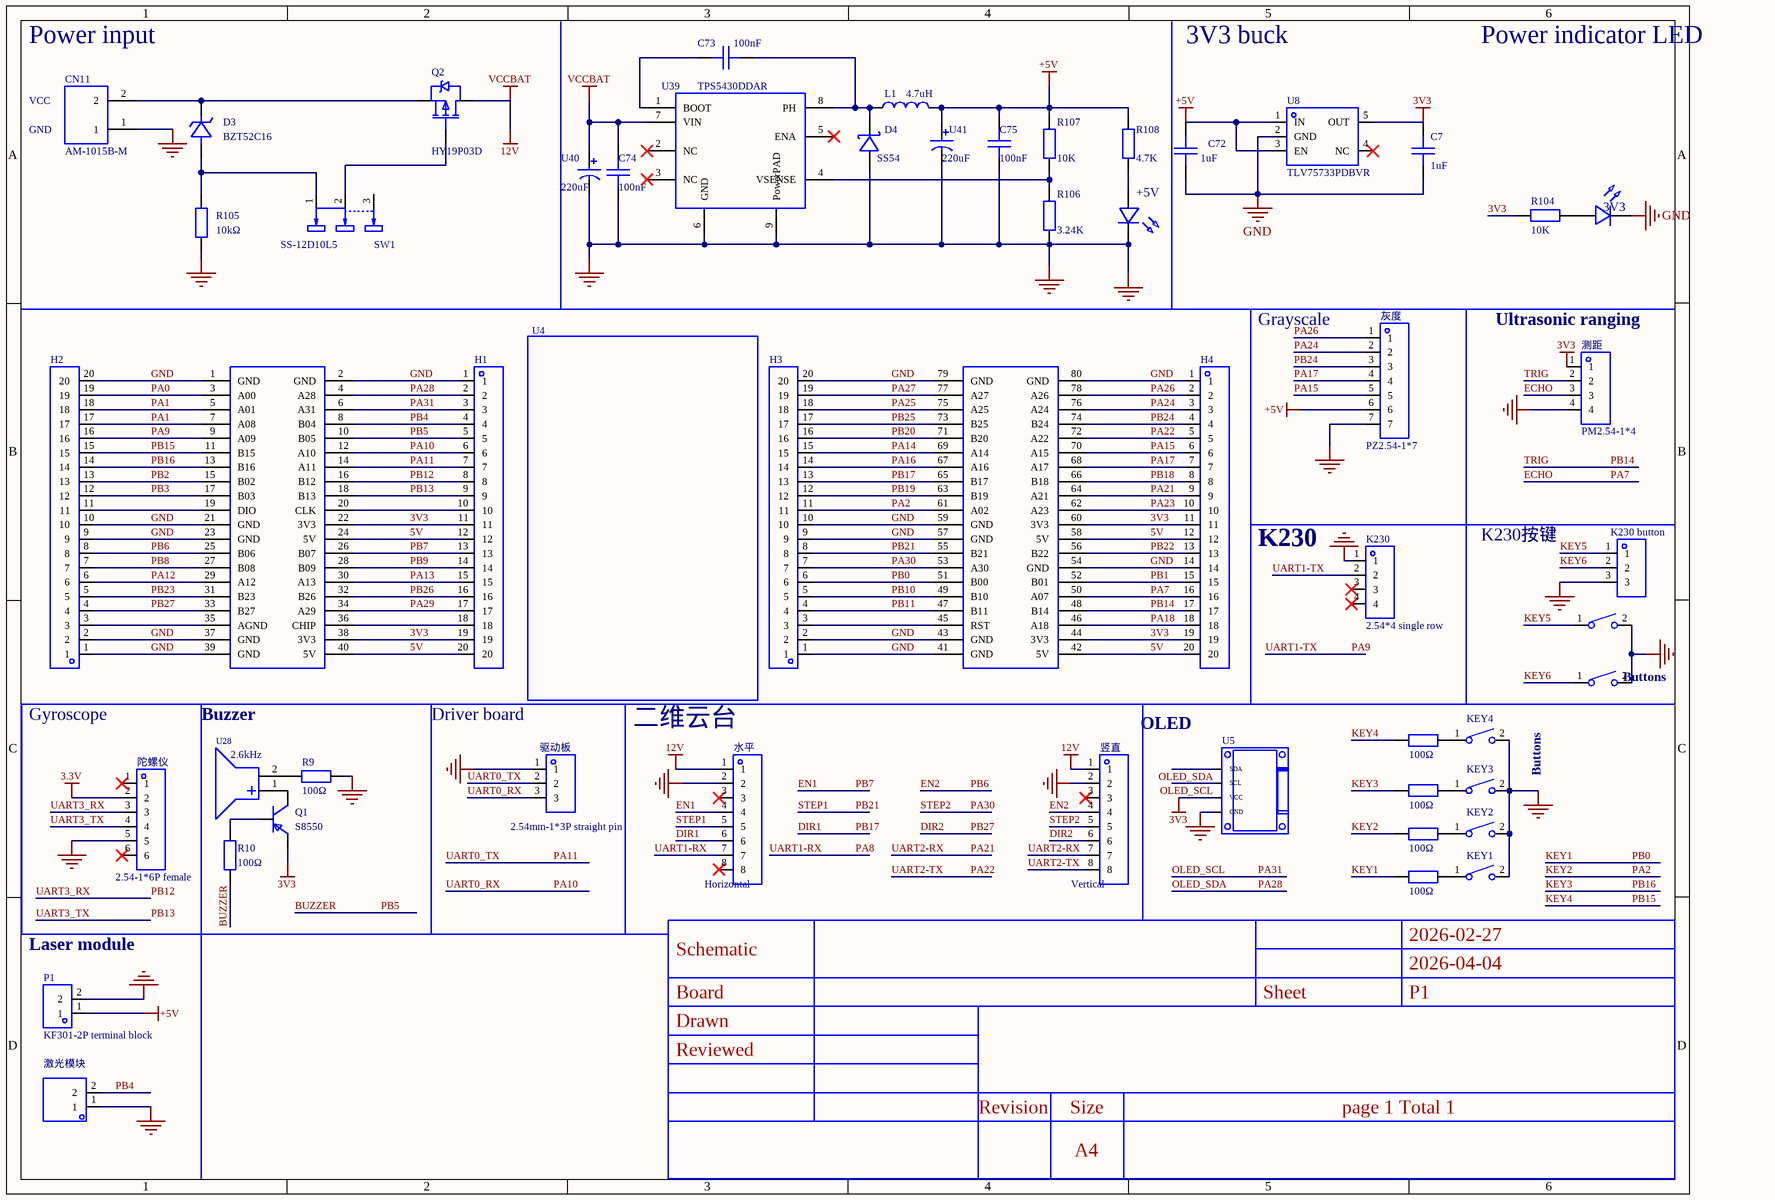
[diagram p0: MISC49883-2.schdoc]
# Altium project MISC49883-3.PrjPcb
1 sheet, 52 parts. Net scope: global (net labels, ports and power ports of the same name join across sheets).
Board file: MISC49883.pcbdoc

## Sheet MISC49883-2.schdoc
size 297 x 209 mm; Version: V1.0; @Project Name: MISC49883; @Page Count: 1; @Update Date: 2026-04-06; @Create Date: 2026-04-06; @Schematic Name: MISC49883; @Page No: 1; @Board Name: MISC49883; @Create Time: 15:17:24; @Update Time: 23:17:25; Size: A4

### Parts
3V3  (no value)  [LED_0603]
+5V  (no value)  [LED_0603]
C7  1uF  [C0603]
C72  1uF  [C0603]
C73  100nF  [C0805]
C74  100nF  [C0805]
C75  100nF  [C0805]
CN11  AM-1015B-M  [CONN-TH_AM-1015B-M]
D3  BZT52C16  [SOD-123_L2.7-W1.6-LS3.7-RD]
D4  SS54  [SMA_L4.4-W2.8-LS5.4-R-RD]
H1  (no value)  [HDR-TH_20P-P2.54-V-M-1]
H2  (no value)  [HDR-TH_20P-P2.54-V-M-1]
H3  (no value)  [HDR-TH_20P-P2.54-V-M-1]
H4  (no value)  [HDR-TH_20P-P2.54-V-M-1]
K230  2.54*4 single row  [HDR-TH_4P-P2.54-V-M-1]
K230按键  K230 button  [HDR-TH_3P-P2.54-V-M]
K230按键1  Tact switch 3*6*2.5  [SW-SMD_L6.0-W3.6-LS8.0]  (value not drawn)
K230按键2  Tact switch 3*6*2.5  [SW-SMD_L6.0-W3.6-LS8.0]  (value not drawn)
KEY1  Tact switch 3*6*2.5  [SW-SMD_L6.0-W3.6-LS8.0]  (value not drawn)
KEY2  Tact switch 3*6*2.5  [SW-SMD_L6.0-W3.6-LS8.0]  (value not drawn)
KEY3  Tact switch 3*6*2.5  [SW-SMD_L6.0-W3.6-LS8.0]  (value not drawn)
KEY4  Tact switch 3*6*2.5  [SW-SMD_L6.0-W3.6-LS8.0]  (value not drawn)
L1  4.7uH  [IND-SMD_L7.3-W6.6]
P1  KF301-2P terminal block  [CONN-TH_XY301V-A-5.0-2P]
Q1  S8550  [SOT-23-3_L2.9-W1.6-P1.90-LS2.8-BR]
Q2  HY19P03D  [TO-252-2_L6.6-W6.1-P4.57-LS9.9-TL-CW]
R9  100Ω  [R0603]
R10  100Ω  [R0603]
R104  10K  [R0603]
R105  10kΩ  [R0603]
R106  3.24K  [R0603]
R107  10K  [R0603]
R108  4.7K  [R0603]
R109  100Ω  [R0603]
R110  100Ω  [R0603]
R111  100Ω  [R0603]
R112  100Ω  [R0603]
SW1  SS-12D10L5  [SW-TH_SS-12D10L5]
U4  (no value)  [COMM-TH_LCKFB-TMX-MSPM0G3507]
U5  (no value)  [0.96OLED_4P]
U8  TLV75733PDBVR  [SOT-23-5_L2.9-W1.6-P0.95-LS2.8-BL]
U28  2.6kHz  [BUZ-TH_BD12.0-P7.60-D0.6-FD]
U39  TPS5430DDAR  [ESOP-8_L4.9-W3.9-P1.27-LS6.0-TL-EP]
U40  220uF  [CAP-SMD_BD6.3-L6.6-W6.6-LS7.2-FD]
U41  220uF  [CAP-SMD_BD6.3-L6.6-W6.6-LS7.2-FD]
水平  Horizontal  [CONN-TH_8P-P2.50-XH2.54-8P]
测距  PM2.54-1*4  [HDR-TH_4P-P2.54-V-F]
激光模块  (no value)  [HDR-TH_2P-P2.54-V-M-1]
灰度  PZ2.54-1*7  [HDR-TH_7P-P2.54-V-M]
竖直  Vertical  [CONN-TH_8P-P2.50-XH2.54-8P]
陀螺仪  2.54-1*6P female  [HDR-TH_6P-P2.54-V-F]
驱动板  2.54mm-1*3P straight pin  [HDR-TH_3P-P2.54-V-M-1]

### Nets
3.3V: 陀螺仪.2
3V3: C7.2 H1.11 H1.19 H4.11 H4.19 Q1.2 R104.1 U4.22(3V3) U4.38(3V3) U4.44(3V3) U4.60(3V3) U5.2(VCC) U8.5(OUT) 测距.1
12V: C74.2 Q2.2(D) U39.7(VIN) U40.1 水平.1 竖直.1  [also labelled VCCBAT]
+5V: C72.2 C75.2 L1.2 P1.1 R107.2 R108.2 U8.1(IN) U8.3(EN) U41.1 灰度.6
GND: 3V3.1(C) +5V.1(C) C7.1 C72.1 C74.1 C75.1 CN11.1 D4.1(A) H1.1 H2.1 H2.2 H2.9 H2.10 H2.20 H3.1 H3.2 H3.9 H3.10 H3.20 H4.1 H4.14 K230.1 K230按键.3 K230按键1.2 K230按键2.2 KEY1.2 KEY2.2 KEY3.2 KEY4.2 P1.2 R9.1 R105.1 R106.1 U4.1(GND) U4.2(GND) U4.21(GND) U4.23(GND) U4.37(GND) U4.39(GND) U4.41(GND) U4.43(GND) U4.54(GND) U4.57(GND) U4.59(GND) U4.79(GND) U4.80(GND) U5.1(GND) U8.2(GND) U39.6(GND) U39.9(PowerPAD) U40.2 U41.2 水平.2 测距.4 激光模块.1 灰度.7 竖直.2 陀螺仪.5 驱动板.1
5V: H1.12 H1.20 H4.12 H4.20 U4.24(5V) U4.40(5V) U4.42(5V) U4.58(5V)
BUZZER: H1.5 R10.2 U4.10(B05)  [also labelled PB5]
DIR1: H3.13 U4.65(B17) 水平.6  [also labelled PB17]
DIR2: H2.4 U4.33(B27) 竖直.6  [also labelled PB27]
ECHO: H4.16 U4.50(A07) 测距.3  [also labelled PA7]
EN1: H1.13 U4.26(B07) 水平.4  [also labelled PB7]
EN2: H2.8 U4.25(B06) 竖直.4  [also labelled PB6]
KEY1: H3.6 R109.2 U4.51(B00)  [also labelled PB0]
KEY2: H3.11 R110.2 U4.61(A02)  [also labelled PA2]
KEY3: H2.14 R111.2 U4.13(B16)  [also labelled PB16]
KEY4: H2.15 R112.2 U4.11(B15)  [also labelled PB15]
KEY5: K230按键.1 K230按键1.1
KEY6: K230按键.2 K230按键2.1
OLED_SCL: H1.3 U4.6(A31) U5.3(SCL)  [also labelled PA31]
OLED_SDA: H1.2 U4.4(A28) U5.4(SDA)  [also labelled PA28]
PA0: H2.19 U4.3(A00)
PA1: H2.17 H2.18 U4.5(A01) U4.7(A08)
PA8: 水平.7  [also labelled UART1-RX]
PA9: H2.16 K230.2 U4.9(A09)  [also labelled UART1-TX]
PA10: H1.6 U4.12(A10) 驱动板.3  [also labelled UART0_RX]
PA11: H1.7 U4.14(A11) 驱动板.2  [also labelled UART0_TX]
PA12: H2.6 U4.29(A12)
PA13: H1.15 U4.30(A13)
PA14: H3.15 U4.69(A14)
PA15: H4.6 U4.70(A15) 灰度.5
PA16: H3.14 U4.67(A16)
PA17: H4.7 U4.68(A17) 灰度.4
PA18: H4.18 U4.46(A18)
PA21: H4.9 U4.64(A21) 竖直.7  [also labelled UART2-RX]
PA22: H4.5 U4.72(A22) 竖直.8  [also labelled UART2-TX]
PA23: H4.10 U4.62(A23)
PA24: H4.3 U4.76(A24) 灰度.2
PA25: H3.18 U4.75(A25)
PA26: H4.2 U4.78(A26) 灰度.1
PA27: H3.19 U4.77(A27)
PA29: H1.17 U4.34(A29)
PA30: H3.7 U4.53(A30) 竖直.5  [also labelled STEP2]
PB1: H4.15 U4.52(B01)
PB2: H2.13 U4.15(B02)
PB3: H2.12 U4.17(B03)
PB4: H1.4 U4.8(B04) 激光模块.2
PB8: H2.7 U4.27(B08)
PB9: H1.14 U4.28(B09)
PB10: H3.5 U4.49(B10)
PB11: H3.4 U4.47(B11)
PB12: H1.8 U4.16(B12) 陀螺仪.3  [also labelled UART3_RX]
PB13: H1.9 U4.18(B13) 陀螺仪.4  [also labelled UART3_TX]
PB14: H4.17 U4.48(B14) 测距.2  [also labelled TRIG]
PB18: H4.8 U4.66(B18)
PB19: H3.12 U4.63(B19)
PB20: H3.16 U4.71(B20)
PB21: H3.8 U4.55(B21) 水平.5  [also labelled STEP1]
PB22: H4.13 U4.56(B22)
PB23: H2.5 U4.31(B23)
PB24: H4.4 U4.74(B24) 灰度.3
PB25: H3.17 U4.73(B25)
PB26: H1.16 U4.32(B26)
Net3V3_2: 3V3.2(A) R104.2
Net+5V_2: +5V.2(A) R108.1
NetC73_1: C73.1 U39.1(BOOT)
NetC73_2: C73.2 D4.2(K) L1.1 U39.8(PH)
NetCN11_2: CN11.2 D3.1(K) Q2.3(S)
NetD3_2: D3.2(A) R105.2 SW1.1
NetH1_10: H1.10 U4.20(CLK)
NetH1_18: H1.18 U4.36(CHIP)
NetH2_3: H2.3 U4.35(AGND)
NetH2_11: H2.11 U4.19(DIO)
NetH3_3: H3.3 U4.45(RST)
NetKEY1_1: KEY1.1 R109.1
NetKEY2_1: KEY2.1 R110.1
NetKEY3_1: KEY3.1 R111.1
NetKEY4_1: KEY4.1 R112.1
NetQ1_1: Q1.1 R10.1
NetQ1_3: Q1.3 U28.1(+)
NetQ2_1: Q2.1(G) SW1.2
NetR9_2: R9.2 U28.2(-)
NetR106_2: R106.2 R107.1 U39.4(VSENSE)

Not connected (* = marked no-connect by the designer): K230 3* 4*; SW1 3; U8 4(NC)*; U39 2(NC)* 3(NC)* 5(ENA)*; 水平 3* 8*; 竖直 3*; 陀螺仪 1* 6*

### Notes on the sheet
- Power input
- 3V3 buck
- Power indicator LED
- VCC
- GND
- (near 灰度) Grayscale
- (near 测距) Ultrasonic ranging
- K230
- Gyroscope
- Buzzer
- Driver board
- OLED
- (near K230按键2) Buttons
- 二维云台
- Buttons
- (near P1) Laser module
- 2026-02-27
- Schematic
- Board
- Sheet
- 2026-04-04
- P1
- Drawn
- Reviewed
- Revision
- Size
- A4
- page 1 Total 1

### Library data of the parts
3V3 +5V = LED_0603-R: Symbol: LED_R; Convert to PCB: yes; 3D Model: dd8257b0d61a4cd7b68939a056e08095; 3D Model Transform: 58.72,29.4,22.03,0,0,0,0,0,0; ModelName: LED-0603_R; Device: LED_0603-R; Add into BOM: yes; Supplier Footprint: 0603; FootprintName: LED_0603
C7 C72 = CAP_0603: SymbolName: Capacitance; ConvertToPcb: yes; ModelId: 05093a7ad16bafb1; ModelName: C0603_L1.6-W0.8-H0.8; ModelTransform: 0,0,0,0,0,0,0,0,0; Device: CAP_0603; Value: 1uF; FootprintName: C0603; AddInBom: yes; Supplier Footprint: 0603
C73-C75 = CC0805KRX7R9BB104: Manufacturer: YAGEO(国巨); AddInBom: yes; Tolerance: ±10%; Voltage Rating: 50V; Temperature Coefficient: X7R; ModelId: 1ba041120af144c991958decab20d241; ModelName: C0805_L2.0-W1.3-H1.3; ModelTransform: 78.74,51.181,0,0,0,0,0,0.0005,0; Device: CC0805KRX7R9BB104; Symbol: CC0805KRX7R9BB104; FootprintName: C0805; LCSC Part Name: 100nF ±10% 50V; SupplierPart: C49678; ManufacturerPart: CC0805KRX7R9BB104; Supplier Footprint: 0805; JLCPCB Part Class: Basic library; Datasheet: https://item.szlcsc.com/datasheet/CC0805KRX7R9BB104/50686.html; Supplier: LCSC; ConvertToPcb: yes; Value: 100nF
CN11 = AM-1015B-M: Manufacturer: AMASS(艾迈斯); AddInBom: yes; ModelId: 5ed58976d70a6d12; ModelTransform: 0,0,0,0,0,0,0,0,0; Device: AM-1015B-M; Symbol: AM-1015B-M; FootprintName: CONN-TH_AM-1015B-M; LCSC Part Name: AMASS(艾迈斯)电源连接器公头AM-1015B-M; SupplierPart: C90631; ManufacturerPart: AM-1015B-M; Supplier Footprint: -; JLCPCB Part Class: Extended library; Datasheet: https://item.szlcsc.com/datasheet/AM-1015B-M/91818.html; Supplier: LCSC; ConvertToPcb: yes; ModelName: CONN-TH_AM-1015B-M
D3 = BZT52C16: Manufacturer: Slkor(萨科微); Symbol: BZT52C16_C707145; AddInBom: yes; Diode Configuration: Discrete; Zener Voltage(Nom): 16V; Reverse Leakage Current (Ir): 100nA; Zener Voltage(Range): 15.3V~17.1V; Pd - Power Dissipation: 500mW; Impedance(Zzt): 40Ω; Operating Junction Temperature Range: -65℃~+150℃; ModelId: ad7e39f9e5534b3c96ffdc5532ebb493; ModelName: SOD-123_L2.7-W1.6-H1.4-LS3.7; ModelTransform: 146.026,62.992,0,180,0,0,0.0005,0,0; Device: BZT52C16; FootprintName: SOD-123_L2.7-W1.6-LS3.7-RD; LCSC Part Name: 独立式 耐压:16V 电流:0.1uA; SupplierPart: C707145; ManufacturerPart: BZT52C16; Supplier Footprint: SOD-123; JLCPCB Part Class: Extended library; Datasheet: https://item.szlcsc.com/datasheet/BZT52C16/744267.html; Supplier: LCSC; ConvertToPcb: yes
D4 = SS54_C22452: Manufacturer: MDD(辰达半导体); AddInBom: yes; Diode Configuration: Discrete; Voltage - Forward(Vf@If): 550mV@5A; Voltage - DC Reverse(Vr): 40V; Current - Rectified: 5A; Reverse Leakage Current (Ir): 1mA@40V; Operating Junction Temperature Range: -55℃~+125℃; ModelId: 686a5d0d1e08618d; ModelTransform: 0,0,0,0,0,0,0,0,0; Device: SS54_C22452; Symbol: SS54_C22452; FootprintName: SMA_L4.4-W2.8-LS5.4-R-RD; LCSC Part Name: 电压:40V 电流:5A; SupplierPart: C22452; ManufacturerPart: SS54; Supplier Footprint: SMA(DO-214AC); JLCPCB Part Class: Basic library; Datasheet: https://item.szlcsc.com/datasheet/SS54/23178.html; Supplier: LCSC; ConvertToPcb: yes; ModelName: SMA_L4.4-W2.8-LS5.4-R-RD
H1-H4 = HDR-M_2.54_1x20P: Symbol: HDR_2.54-1x20P; ConvertToPcb: yes; ModelId: f68709be121d406db68b06f32a595389; ModelName: HDR-M-2.54_1x20; ModelTransform: 1999.996,100,0,0,0,0,0,2.48,-118.11; Device: HDR-M_2.54_1x20P; FootprintName: HDR-TH_20P-P2.54-V-M-1; AddInBom: yes; SupplierPart: C50981; Supplier Footprint: 插件
K230 = 2.54*4单排: AddInBom: yes; ModelId: e2e03939c192453cba872779c0cb6390; ModelTransform: 400.039,100,0,0,0,0,0,0,-118.11; Device: 2.54*4 single row; Symbol: 2.54*4 single row; FootprintName: HDR-TH_4P-P2.54-V-M-1; LCSC Part Name: 2.54*4单排; SupplierPart: C9900016163; ManufacturerPart: 2.54*4单排; Supplier Footprint: 2.54x4; JLCPCB Part Class: Extended library; Supplier: LCSC; ConvertToPcb: yes; ModelName: HDR-TH_4P-P2.54-V-M-1
K230按键 = HDR-M_2.54_1x3P: AddInBom: yes; ModelId: bb473b6d38ff42a99216a4fcdbdcc4cb; ModelName: HDR-TH_3P-P2.54-M-LI-1X3P; ModelTransform: 300.03877,100,0,0,0,0,0,0,-118.11; Device: HDR-M_2.54_1x3P; Symbol: HDR-M_2.54_1x3P; FootprintName: HDR-TH_3P-P2.54-V-M; ConvertToPcb: yes; SupplierPart: C2937625; Supplier Footprint: 插件; JLCPCB Part Class: Extended library
K230按键1 K230按键2 KEY1-KEY4 = 轻触按键3*6*2.5: AddInBom: yes; ModelId: 5cda64a5897044e48badc24f5aa7d420; ModelName: SW-SMD_L6.0-W3.6-H2.5-LS8.0; ModelTransform: 314.96,141.732,0,0,0,0,0,0,0; Device: Tact switch 3*6*2.5; Symbol: Tact switch 3*6*2.5; FootprintName: SW-SMD_L6.0-W3.6-LS8.0; LCSC Part Name: 轻触按键3*6*2.5; SupplierPart: C9900013040; ManufacturerPart: 轻触按键3*6*2.5; Supplier Footprint: KEY; JLCPCB Part Class: Extended library; Supplier: LCSC; ConvertToPcb: yes
L1 = MCS0630-4R7MPY1: Manufacturer: PSA(信昌电陶); AddInBom: yes; Tolerance: ±20%; Rated Current: 5.5A; Saturation Current (Isat): 7A; DC Resistance (DCR): 37mΩ; ModelId: f365aa58eec94c2a8dfc1404764b7425; ModelName: IND-SMD_L7.1-W6.6-H2.8; ModelTransform: 279.527,259.842,0,0,0,0,0.0005,0,0; Device: MCS0630-4R7MPY1; Symbol: MCS0630-4R7MPY1; FootprintName: IND-SMD_L7.3-W6.6; LCSC Part Name: 4.7uH ±20% 7A; SupplierPart: C2937097; ManufacturerPart: MCS0630-4R7MPY1; Supplier Footprint: 0630; JLCPCB Part Class: Extended library; Datasheet: https://atta.szlcsc.com/upload/public/pdf/source/20220121/EA6E6E6F70ED7BAE67EC293805EAAACB.pdf; Supplier: LCSC; ConvertToPcb: yes; Value: 4.7uH
P1 = KF301-2P接线端子: AddInBom: yes; ModelId: ef7ead88b0f2448d904975b26718870f; ModelTransform: 417.322,299.212,0,0,0,0,11.811,-7.835,-157.48; Device: KF301-2P terminal block; Symbol: KF301-2P terminal block; FootprintName: CONN-TH_XY301V-A-5.0-2P; LCSC Part Name: KF301-2P接线端子; SupplierPart: C9900016950; ManufacturerPart: KF301-2P接线端子; Supplier Footprint: CK301-2P; JLCPCB Part Class: Extended library; Supplier: LCSC; ConvertToPcb: yes; ModelName: CONN-TH_XY301V-A-5.0-2P
Q1 = S8550_C105432: Manufacturer: CJ(江苏长电/长晶); AddInBom: yes; Transistor Type: PNP; Collector Current (Ic): 500mA; Collector-Emitter Breakdown Voltage (Vceo): 25V; Power Dissipation (Pd): 300mW; DC Current Gain (hFE@Ic,Vce): 120@50mA,1V; Transition Frequency (fT): 150MHz; Collector Cut-Off Current (Icbo): 100nA; Collector-Emitter Saturation Voltage (VCE(sat)@Ic,Ib): 600mV@500mA,50mA; ModelId: 89cb27a44ab2466697082bb9fd73a7d0; ModelName: SOT-23-3L_L2.9-W1.6-H1.1-LS2.8-P0.95; ModelTransform: 114.173,110.236,0,90,0,0,0,0,0; Device: S8550_C105432; Symbol: S8550_C105432; FootprintName: SOT-23-3_L2.9-W1.6-P1.90-LS2.8-BR; LCSC Part Name: S8550(RANGE:120-200) L档120-200; SupplierPart: C105432; ManufacturerPart: S8550; Supplier Footprint: SOT-23; JLCPCB Part Class: Basic library; Datasheet: https://atta.szlcsc.com/upload/public/pdf/source/20171228/C164891_15144412930301213894.pdf; Supplier: LCSC; ConvertToPcb: yes; Operating Temperature: -
Q2 = HY19P03D: Manufacturer: HUAYI(华羿微); AddInBom: yes; Type: P-channel; Drain Source Voltage (Vdss): 30V; Continuous Drain Current (Id): 90A; Power Dissipation (Pd): 50W; Drain Source On Resistance (RDS(on)@Vgs,Id): 6mΩ@10V,45A; Gate Threshold Voltage (Vgs(th)@Id): 3V@250uA; ModelId: ce57f84d66384067af8a68020b6de06d; ModelName: TO-252-2L-3P_L6.6-W6.1-H2.3-LS10.1-P4.6; ModelTransform: 259.842,390.52442,0,270,0,0,38.027,-0.598,0; Device: HY19P03D; Symbol: HY19P03D; FootprintName: TO-252-2_L6.6-W6.1-P4.57-LS9.9-TL-CW; LCSC Part Name: P沟道 耐压:30V 电流:90A; SupplierPart: C122492; ManufacturerPart: HY19P03D; Supplier Footprint: TO-252-2; JLCPCB Part Class: Extended library; Datasheet: https://atta.szlcsc.com/upload/public/pdf/source/20170728/C122492_1501225751911848809.pdf; Supplier: LCSC; ConvertToPcb: yes
R9 R10 R104 R106-R108 = Res_0603: Symbol: Resistor; ConvertToPcb: yes; ModelId: 4a58f241193a162b; ModelTransform: 0,0,0,0,0,0,0,0,0; Device: Res_0603; FootprintName: R0603; AddInBom: yes; Supplier Footprint: 0603; ModelName: R0603
  R9 R10: Value: 100Ω
  R104 R107: Value: 10K
  R106: Value: 3.24K
  R108: Value: 4.7K
R105 = 0603WAF1002T5E: Manufacturer: UNI-ROYAL(厚声); AddInBom: yes; Tolerance: ±1%; Power(Watts): 100mW; Overload Voltage (Max): 75V; Temperature Coefficient: ±100ppm/℃; ModelId: fc143cca1e79419f9cd78b61e9279f08; ModelTransform: 31.8897,63.7794,0,90,0,0,0,0,0; Device: 0603WAF1002T5E; Symbol: 0603WAF1002T5E; Supplier: LCSC; Manufacturer Part: 0603WAF1002T5E; Supplier Part: C25804; Value: 10kΩ; JLCPCB Part Class: Basic library; FootprintName: R0603; LCSC Part Name: 厚膜电阻 10kΩ ±1% 100mW; Supplier Footprint: 0603; Datasheet: https://atta.szlcsc.com/upload/public/pdf/source/20200306/C422600_1E6D84923E4A46A82E41ADD87F860B5C.pdf; ConvertToPcb: yes; Type: Thick film resistor; Operating Temperature Range: -55℃~+155℃; ModelName: R0603
R109-R112 = 0603WAF1000T5E: Manufacturer: UNI-ROYAL(厚声); AddInBom: yes; Tolerance: ±1%; Power(Watts): 100mW; Overload Voltage (Max): 75V; Temperature Coefficient: ±200ppm/℃; ModelId: fc143cca1e79419f9cd78b61e9279f08; ModelTransform: 31.8897,63.7794,0,90,0,0,0,0,0; Device: 0603WAF1000T5E; Symbol: 0603WAF1000T5E; FootprintName: R0603; LCSC Part Name: 100Ω ±1% 100mW 厚膜电阻; SupplierPart: C22775; ManufacturerPart: 0603WAF1000T5E; Supplier Footprint: 0603; JLCPCB Part Class: Basic library; Datasheet: https://atta.szlcsc.com/upload/public/pdf/source/20200306/C422600_1E6D84923E4A46A82E41ADD87F860B5C.pdf; Supplier: LCSC; ConvertToPcb: yes; Type: Thick film resistor; Value: 100Ω; Operating Temperature Range: -55℃~+155℃; ModelName: R0603
SW1 = SS-12D10L5: Manufacturer: XKB Connectivity(中国星坤); AddInBom: yes; Circuit: SPDT; Actuator Style: Rectangular post; Pin Style: PC pin; Switch Length: 13mm; Switch Width: 6.8mm; Switch Height: 6.4mm; Actuator Color: Black; Current Rating (DC): 3A; Voltage Rating (DC): 125V; Mechanical Life: 1万次; ModelId: c49f07a32c154ec8ad7cf47670a53981; ModelName: SW-TH_L13.0-W6.8-H6.4-P4.7; ModelTransform: 511.81,267.716,0,0,0,0,0,0,-275.591; Device: SS-12D10L5; Symbol: SS-12D10L5; FootprintName: SW-TH_SS-12D10L5; LCSC Part Name: 柄长5mm 直插双档 滑动开关; SupplierPart: C319012; ManufacturerPart: SS-12D10L5; Supplier Footprint: 插件; JLCPCB Part Class: Extended library; Datasheet: https://atta.szlcsc.com/upload/public/pdf/source/20211009/D6412F37AABE6F9459A6EE7FA4DAEADB.pdf; Supplier: LCSC; ConvertToPcb: yes; Mounting Style: Through-hole; Current Rating (AC): 3A; Voltage Rating (AC): 125V; Operating Temperature: -40℃~+85℃
U4 = LCKFB-TMX-MSPM0G3507: Manufacturer: 立创开发板; AddInBom: yes; ModelId: 8c2b7ba131d4412eae9a4354ab816d50; ModelTransform: 1769.654,2753.608,0,0,0,0,0,-56.102,-236.22; Device: LCKFB-TMX-MSPM0G3507; Symbol: LCKFB-TMX-MSPM0G3507; LCSC Part Name: 立创·天猛星MSPM0G3507开发板 5件套; FootprintName: COMM-TH_LCKFB-TMX-MSPM0G3507; SupplierPart: C42378531; ManufacturerPart: LCKFB-TMX-MSPM0G3507; Supplier Footprint: -; Datasheet: https://atta.szlcsc.com/upload/public/pdf/source/20241209/800332349277522348D9357AB5109808.pdf; Supplier: LCSC; ConvertToPcb: yes; ModelName: COMM-TH_LCKFB-TMX-MSPM0G3507
U5 = 0.96OLED模块_4P: Device: 0.96OLED module_4P; ConvertToPcb: yes; ModelId: 79c000fdb68d45a296c2e9bedf4f9055; ModelTransform: 1393.69792,1318.895,0,0,0,0,0,-560.079,-137.795; SymbolName: 0.96OLED module_4P; FootprintName: 0.96OLED_4P; AddInBom: yes; Supplier Footprint: 插件; ModelName: 0.96OLED_4P
U8 = TLV75733PDBVR: Manufacturer: TI(德州仪器); AddInBom: yes; Output Type: Fixed; Maximum Input Voltage: 5.5V; Output Voltage: 3.3V; Output Current: 1A; Power Supply Rejection Ratio (PSRR): 52dB; Dropout Voltage: 475mV@(1A); Output Polarity: Positive; Number of Outputs: 1; ModelId: 018c57e721114987ae90467fe9f1d259; ModelTransform: 114.96,110.236,0,0,0,0,0,0,0; Device: TLV75733PDBVR; Symbol: TLV75733PDBVR; FootprintName: SOT-23-5_L2.9-W1.6-P0.95-LS2.8-BL; LCSC Part Name: 具有使能功能的 1A、低 IQ、高精度、低压降稳压器; SupplierPart: C485517; ManufacturerPart: TLV75733PDBVR; Supplier Footprint: SOT-23-5; JLCPCB Part Class: Extended library; Supplier: LCSC; ConvertToPcb: yes; Feature: ESD protection; surge protection; low ESR; thermal shutdown (TSD); undervoltage lockout; overcurrent protection (OCP); with enable; Operating Temperature: -40℃~+125℃@(Tj); ModelName: SOT-23-5_L2.9-W1.6-P0.95-LS2.8-BL
U28 = HYE1206-05ST: Manufacturer: HYDZ(华宇); AddInBom: yes; Sound Pressure Level (SPL): 80dB@5V,10cm; ModelId: 16ab50e14c5b4f2c986c135bdba60e37; ModelName: BUZ-TH_D12.0-H9.5-P7.60; ModelTransform: 472.44,472.176,0,90,0,0,-0.787,0,-177.165; Device: HYE1206-05ST; Symbol: HYE1206-05ST; Supplier: LCSC; Supplier Part: C17701079; Manufacturer Part: HYE1206-05ST; FootprintName: BUZ-TH_BD12.0-P7.60-D0.6-FD; LCSC Part Name: 有源蜂鸣器HYE1206-05ST; Supplier Footprint: 插件,D=7.6mm; Datasheet: https://atta.szlcsc.com/upload/public/pdf/source/20230912/EF3443D3A1B92F495A3EE65EE7F2091F.pdf; ConvertToPcb: yes; Value: 2.6kHz
U39 = TPS5430DDAR: Manufacturer: TI(德州仪器); AddInBom: yes; Function: Buck; Output Type: Adjustable; Input Voltage: 5.5V~36V; Output Voltage: 1.221V~32.04V; Output Current (Max): 3A; Switching Frequency: 500kHz; Synchronous Rectification: No; Number of Outputs: 1; Switch tube (built-in/external): Built-in; ModelId: 9497d4a38dde85eb; ModelTransform: 0,0,0,0,0,0,0,0,0; Device: TPS5430DDAR; Symbol: TPS5430DDAR; FootprintName: ESOP-8_L4.9-W3.9-P1.27-LS6.0-TL-EP; LCSC Part Name: 降压 3A 36V; SupplierPart: C9864; ManufacturerPart: TPS5430DDAR; Supplier Footprint: SOIC-8-EP; JLCPCB Part Class: Basic library; Supplier: LCSC; ConvertToPcb: yes; Operating Temperature: -40℃~+125℃@(TJ); Topology: Buck; ModelName: ESOP-8_L4.9-W3.9-P1.27-LS6.0-TL-EP
U40 U41 = 220uF: AddInBom: yes; ModelId: ee2f2020be7dbf1f; ModelTransform: 0,0,0,0,0,0,0,0,0; Device: 220uF; Symbol: 220UF; FootprintName: CAP-SMD_BD6.3-L6.6-W6.6-LS7.2-FD; LCSC Part Name: 220uF; SupplierPart: C2941234; ManufacturerPart: 220uF; Supplier Footprint: -SMD6.3/5.8; JLCPCB Part Class: Extended library; Supplier: LCSC; ConvertToPcb: yes; ModelName: CAP-SMD_BD6.3-L6.6-W6.6-LS7.2-FD
水平 = XH2.54-8P 直插: Manufacturer Part: 水平; Device: XH2.54-8P through-hole; AddInBom: yes; ModelId: 385b1d4b778b4141959d674ea048df76; ModelTransform: 885.825,228.346,0,180,0,0,0.591,-19.094,-137.795; Symbol: XH2.54-8P through-hole; FootprintName: CONN-TH_8P-P2.50-XH2.54-8P; LCSC Part Name: XH2.54-8P 直插; SupplierPart: C9900000730; Supplier Footprint: TH-8_5.8X22.5X2.54P; JLCPCB Part Class: Extended library; Supplier: LCSC; ConvertToPcb: yes; ModelName: CONN-TH_8P-P2.50-XH2.54-8P
测距 = PM2.54-1*4: Manufacturer: ZHOURI(洲日); AddInBom: yes; Holes Structure: 1x4P; Pitch: 2.54mm; Circular Hole / Square Hole: Square hole; Number of Positions: 4P; Current Rating: 2.5A; Holes Direction: Top; ModelId: d187812051054f85879fcaa51a310d8e; ModelTransform: 419.6842,98.464,0,0,0,0,0,0,-118.11; Device: PM2.54-1*4; Symbol: PM2.54-1*4; FootprintName: HDR-TH_4P-P2.54-V-F; LCSC Part Name: 间距:2.54mm 1x4P 直插; SupplierPart: C5116530; ManufacturerPart: PM2.54-1*4; Supplier Footprint: 插件,P=2.54mm; JLCPCB Part Class: Extended library; Datasheet: https://item.szlcsc.com/datasheet/PM2.54-1*4/5692947.html; Supplier: LCSC; ConvertToPcb: yes; Row Spacing: 2.54mm; Mounting Type: Through-hole; Number of Rows: Single row; Insulation Height: 8.5mm; Operating Temperature: -40℃~+105℃; ModelName: HDR-TH_4P-P2.54-V-F
激光模块 = HDR-M_2.54_1x2P: Symbol: 210S-1*2P L=11.6MMGold-plated black; ConvertToPcb: yes; ModelId: 79b2e9f2d70a4d68a1b7098f27c6d4c5; ModelName: HDR-M-2.54_1x2; ModelTransform: 200,100,0,0,0,0,0,0,-118.11; Device: HDR-M_2.54_1x2P; FootprintName: HDR-TH_2P-P2.54-V-M-1; AddInBom: yes; SupplierPart: C124375; Supplier Footprint: 插件; JLCPCB Part Class: Extended library
灰度 = PZ2.54-1*7: Manufacturer: ZHOURI(洲日); AddInBom: yes; Pin Structure: 1x7P; Pitch: 2.54mm; Circluar Pins/Square Pins: Square pin; Current Rating: 2.5A; ModelId: 3f496cdc752348c6a5e9157bbaceaf96; ModelName: HDR-TH_7P-P2.54-M-LI-1X7P; ModelTransform: 690.1561,98.425,0,0,0,0,0,0,-118.11; Device: PZ2.54-1*7; Symbol: PZ2.54-1*7; FootprintName: HDR-TH_7P-P2.54-V-M; LCSC Part Name: 1x7P 间距:2.54mm 方针 直插; SupplierPart: C5360900; ManufacturerPart: PZ2.54-1*7; Supplier Footprint: 插件,P=2.54mm; JLCPCB Part Class: Extended library; Datasheet: https://item.szlcsc.com/datasheet/PZ2.54-1*7/6180459.html; Supplier: LCSC; ConvertToPcb: yes; Mounting Type: Through-hole; Number of Rows: Single row; Number of Pins: 7P; Length of Mating Pin: 6mm; Insulation Height: 2.54mm; Length of End Connection Pin: 3mm; Contact Material: Brass; Contact Plating: Gold; Operating Temperature: -40℃~+105℃
竖直 = XH2.54-8P 直插: Manufacturer Part: 竖直; Device: XH2.54-8P through-hole; AddInBom: yes; ModelId: 385b1d4b778b4141959d674ea048df76; ModelTransform: 885.825,228.346,0,180,0,0,0.591,-19.094,-137.795; Symbol: XH2.54-8P through-hole; FootprintName: CONN-TH_8P-P2.50-XH2.54-8P; LCSC Part Name: XH2.54-8P 直插; SupplierPart: C9900000730; Supplier Footprint: TH-8_5.8X22.5X2.54P; JLCPCB Part Class: Extended library; Supplier: LCSC; ConvertToPcb: yes; ModelName: CONN-TH_8P-P2.50-XH2.54-8P
陀螺仪 = 2.54-1*6P母: Manufacturer: BOOMELE(博穆精密); Symbol: Header-Female-2.54_1x6; AddInBom: yes; Holes Structure: 1x6P; Pitch: 2.54mm; Circular Hole / Square Hole: Square hole; Number of Positions: 6P; Current Rating: 3A; Holes Direction: Top; PIN Length: 3.3mm; ModelId: 0f5bcf94dcda47d085f24cdca1696fe9; ModelTransform: 619.684,94.488,0,0,0,0,0,0,-125.984; Device: 2.54-1*6P female; FootprintName: HDR-TH_6P-P2.54-V-F; LCSC Part Name: 1x6P 间距:2.54mm 直插; SupplierPart: C40877; ManufacturerPart: 2.54-1*6P母; Supplier Footprint: 插件,P=2.54mm; JLCPCB Part Class: Extended library; Datasheet: https://item.szlcsc.com/datasheet/2.54-1*6P%25E6%25AF%258D/41861.html; Supplier: LCSC; ConvertToPcb: yes; Row Spacing: -; Mounting Type: Through-hole; Number of Rows: Single row; Voltage Rating (Max): -; Insulation Height: -; Contact Material: Brass; Contact Plating: -; Operating Temperature: -40℃~+105℃; Supplementary Features: -; ModelName: HDR-TH_6P-P2.54-V-F
驱动板 = 2.54mm-1*3P 直针: AddInBom: yes; ModelId: 94a8ffe137b6410295cb18cd3ffd99db; ModelName: HDR-M-2.54_1x3; ModelTransform: 299.9994,100,0,0,0,0,0,0,-118.11; Device: 2.54mm-1*3P straight pin; Symbol: 2.54MM-1*3P straight pin; FootprintName: HDR-TH_3P-P2.54-V-M-1; LCSC Part Name: 2.54mm-1*3P 直针; SupplierPart: C9900025313; ManufacturerPart: 2.54mm-1*3P 直针; Supplier Footprint: 2.54-180-3P; JLCPCB Part Class: Extended library; Supplier: LCSC; ConvertToPcb: yes